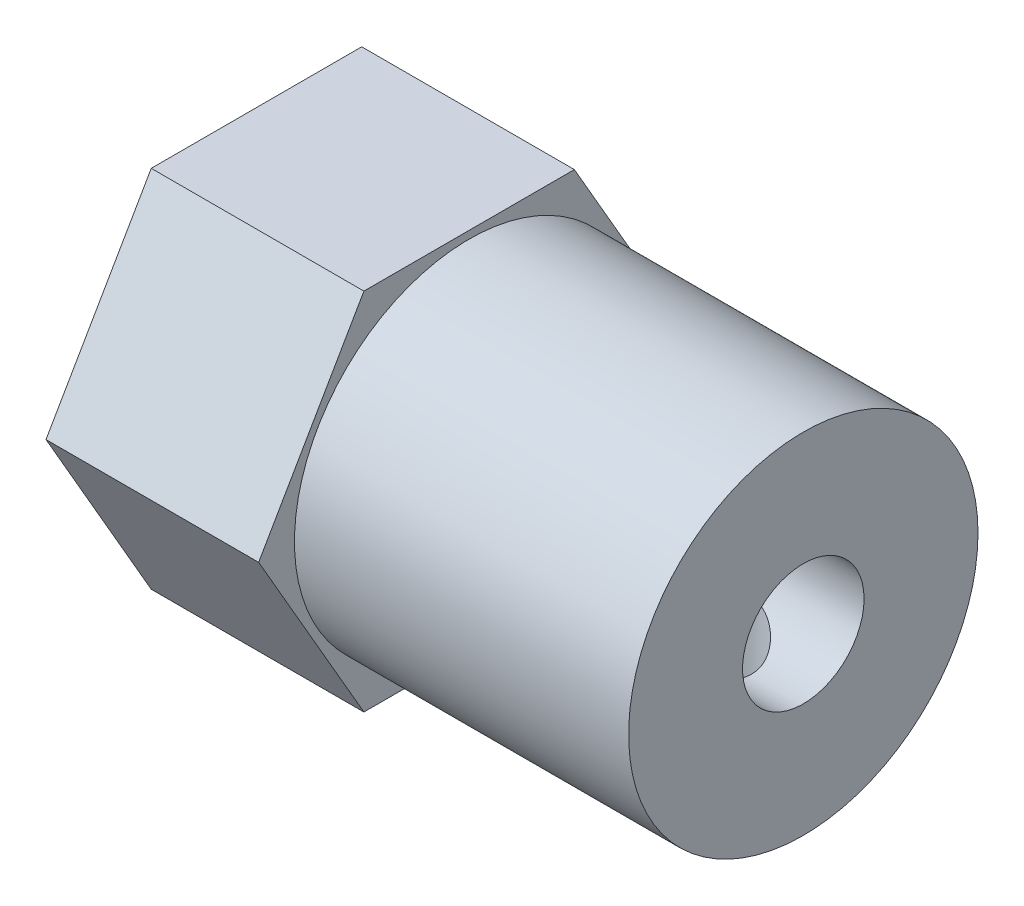
SolidWorks part; units mm, degrees
ref_plane "Front Plane" through (0, 0, 0) normal (0, 0, 1) x (1, 0, 0)
ref_plane "Top Plane" through (0, 0, 0) normal (0, 1, 0) x (1, 0, 0)
ref_plane "Right Plane" through (0, 0, 0) normal (1, 0, 0) x (0, 0, -1)
other "Configuration Table"
sketch "Sketch1" plane through (0, 0, 0) normal (1, 0, 0) x (0, 0, -1)
  line L1 (6.9282, 0) -> (3.4641, 6)
  line L2 (3.4641, 6) -> (-3.4641, 6)
  line L3 (-3.4641, 6) -> (-6.9282, 0)
  line L4 (-6.9282, 0) -> (-3.4641, -6)
  line L5 (-3.4641, -6) -> (3.4641, -6)
  line L6 (3.4641, -6) -> (6.9282, 0)
  circle A0 centre (0, 0) radius 6 construction
  dimension "D1" = 12
extrude "Boss-Extrude1" add sketch "Sketch1" along normal blind 7
sketch "Sketch2" plane through (7, 0, 0) normal (1, 0, 0) x (0, 0, -1)
  circle A0 centre (0, 0) radius 5.75
  dimension "D1" = 11.5
extrude "Boss-Extrude2" add sketch "Sketch2" along normal blind 11
sketch "Sketch3" plane through (18, 0, 0) normal (1, 0, 0) x (0, 0, -1)
  circle A0 centre (0, 0) radius 2
  dimension "D1" = 4
extrude "Cut-Extrude1" cut sketch "Sketch3" against normal blind 10
hole_wizard "M4 Tapped Hole1" positions "Sketch4" profile "Sketch5" tap size "M4" standard "GB" end condition up to next
sketch "Sketch4" plane through (0, 0, 0) normal (-1, 0, 0) x (0, 0, 1)
  point P0 (0, 0)
sketch "Sketch5" plane through (0, 0, 0) normal (0, 1, 0) x (0, 0, 1)
  line L0 (0, 0) -> (0, 8)
  line L1 (0, 8) -> (1.65, 8)
  line L2 (1.65, 8) -> (1.65, 0.375)
  line L3 (1.65, 0.375) -> (2.025, 0)
  line L5 (2.025, 0) -> (0, 0)
  line L6 (-1.65, 0.375) -> (-2.025, 0) construction
  line L11 (0, -6.35) -> (0, 107.95) construction
  dimension "通孔螺纹孔钻头直径" = 3.3
  dimension "通孔螺纹孔钻头深度" = 8
  dimension "近端锥形沉头孔直径" = 4.05
  dimension "近端锥形沉头孔角度" = 90
cosmetic thread "Cosmetic thread1" parameters "D2"=4
sketch "Sketch6" plane through (0, 0, 0) normal (0, 1, 0) x (1, 0, 0)
  line L0 (18, -5.75) -> (18, 5.75) construction
  circle A0 centre (14.8, 0) radius 1.5
  dimension "D1" = 3
  dimension "D2" = 3.2
extrude "Cut-Extrude2" cut sketch "Sketch6" against normal through all
